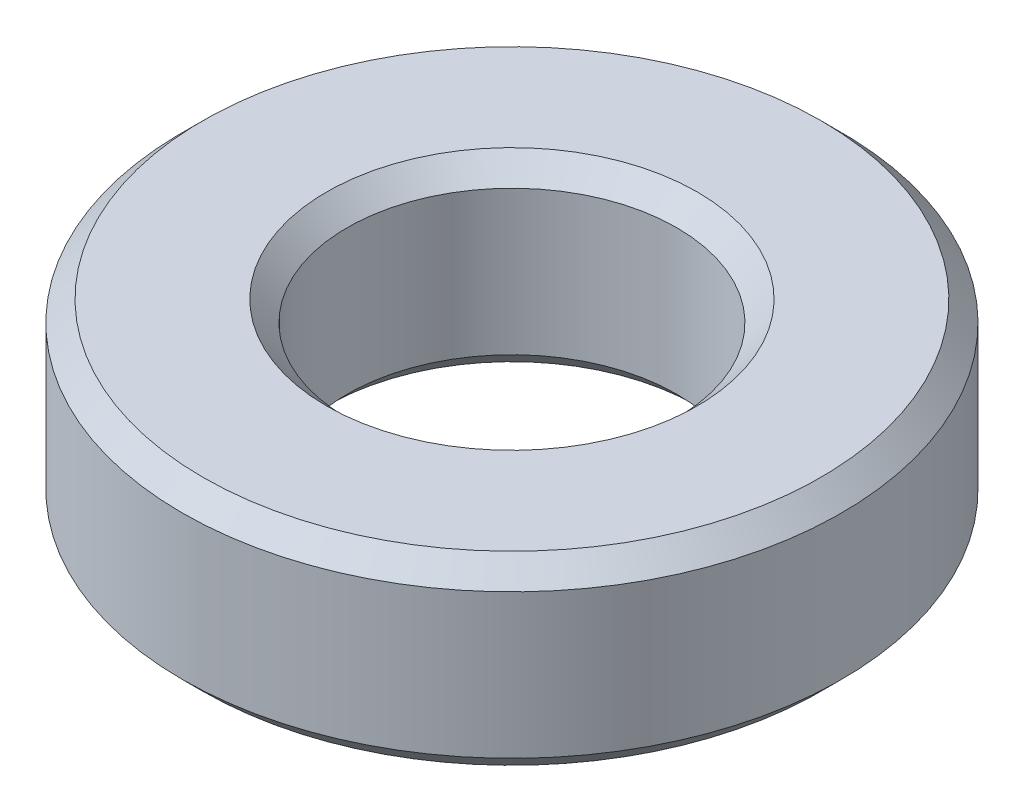
SolidWorks part; units mm, degrees
material "20#"
ref_plane "Front Plane" through (0, 0, 0) normal (0, 0, 1) x (1, 0, 0)
ref_plane "Top Plane" through (0, 0, 0) normal (0, 1, 0) x (1, 0, 0)
ref_plane "Right Plane" through (0, 0, 0) normal (1, 0, 0) x (0, 0, -1)
sketch "Sketch1" plane through (0, 0, 0) normal (0, 1, 0) x (1, 0, 0)
  circle A0 centre (0, 0) radius 4
  circle A1 centre (0, 0) radius 8
  dimension "D1" = 16
  dimension "D2" = 8
extrude "Boss-Extrude1" add sketch "Sketch1" along normal blind 4.5
chamfer "Chamfer1" distance 0.5 angle 45 4 edges at (0, 0, 4) (0, 4.5, 4) (0, 0, 8) (0, 4.5, 8)
